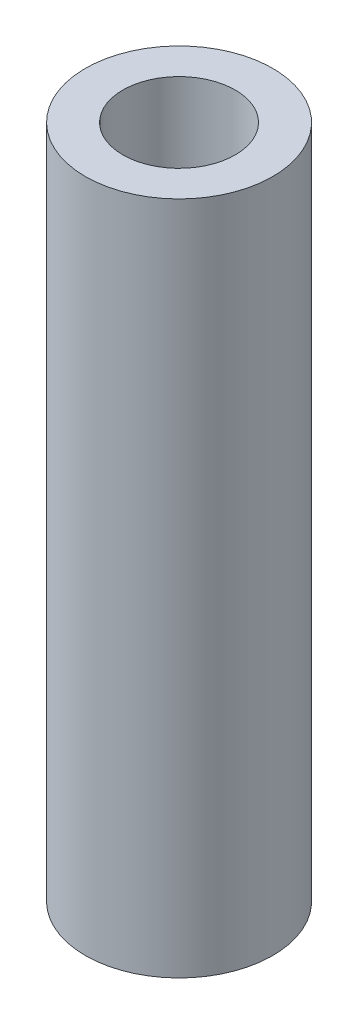
from build123d import *

# Parameters (mm, degrees)
SKETCH_1_R      = 2.5
SKETCH_1_R_2    = 1.5
EXTRUDE_1_DEPTH = 18


with BuildPart() as part:
    # 草图1 → 凸台-拉伸1 (new body)
    with BuildSketch(Plane(origin=(0, 0, 0), x_dir=(1, 0, 0), z_dir=(0, 1, 0))):
        with Locations(Location((0, 0, 0), (0, 0, 270))):
            Circle(SKETCH_1_R)
        with Locations(Location((0, 0, 0), (0, 0, 270))):
            Circle(SKETCH_1_R_2, mode=Mode.SUBTRACT)
    extrude(amount=EXTRUDE_1_DEPTH)


solid = part.part
